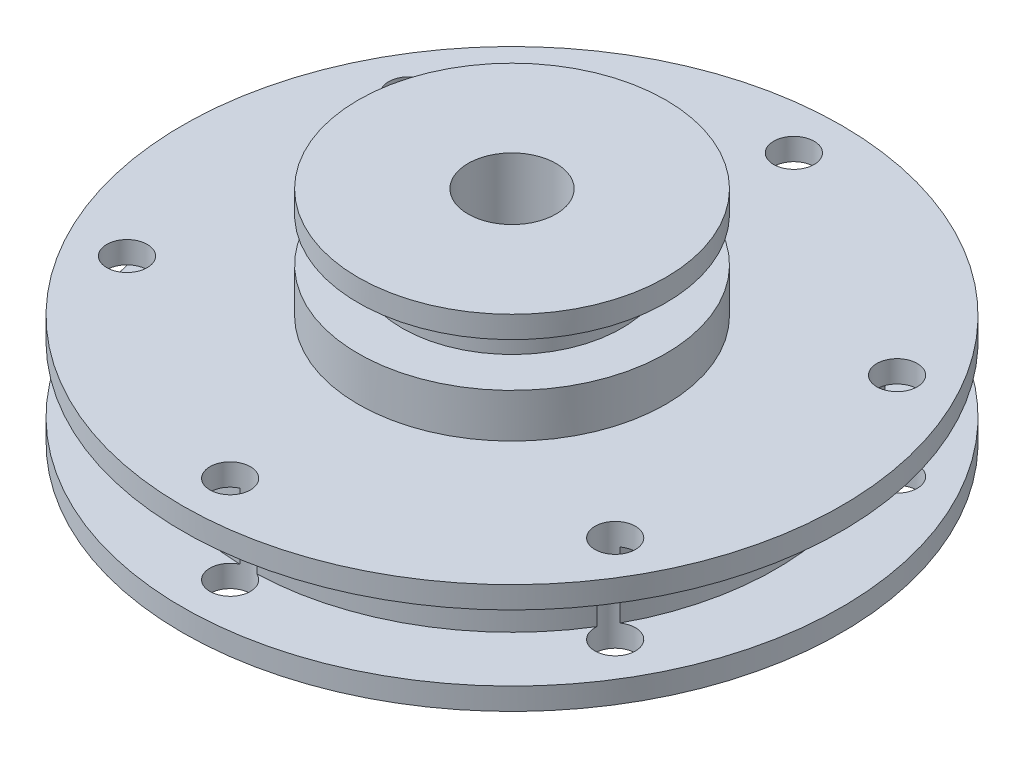
SolidWorks part; units mm, degrees
ref_plane "Front Plane" through (0, 0, 0) normal (0, 0, 1) x (1, 0, 0)
ref_plane "Top Plane" through (0, 0, 0) normal (0, 1, 0) x (1, 0, 0)
ref_plane "Right Plane" through (0, 0, 0) normal (1, 0, 0) x (0, 0, -1)
other "Configuration Table"
sketch "Sketch1" plane through (0, 0, 0) normal (0, 1, 0) x (1, 0, 0)
  circle A0 centre (0, 0) radius 15
  dimension "D1" = 30
extrude "Boss-Extrude1" add sketch "Sketch1" along normal blind 5
sketch "Sketch2" plane through (0, 0, 0) normal (0, 0, 1) x (1, 0, 0)
  line L0 (15, 0) -> (15, 5) construction
  line L1 (15, 4) -> (12, 4)
  line L2 (15, 4) -> (15, 1)
  line L3 (15, 1) -> (12, 1)
  line L4 (12, 4) -> (12, 1)
  line L5 (15, 5) -> (-15, 5) construction
  line L6 (0, 0) -> (0, 8.3794) construction
  line L7 (-15, 0) -> (15, 0) construction
  dimension "D1" = 3
  dimension "D2" = 3
  dimension "D3" = 1
revolve "Cut-Revolve1" cut sketch "Sketch2" angle 360 about L6
sketch "Sketch3" plane through (0, 5, 0) normal (0, 1, 0) x (1, 0, 0)
  circle A0 centre (0, 0) radius 7
  dimension "D1" = 14
extrude "Boss-Extrude2" add sketch "Sketch3" along normal blind 5
sketch "Sketch4" plane through (0, 0, 0) normal (0, 0, 1) x (1, 0, 0)
  line L0 (7, 5) -> (7, 10) construction
  line L1 (7, 9) -> (5, 9)
  line L2 (7, 9) -> (7, 7)
  line L3 (7, 7) -> (5, 7)
  line L4 (5, 9) -> (5, 7)
  line L5 (7, 10) -> (-7, 10) construction
  line L6 (0, 0) -> (0, 9.3794) construction
  dimension "D1" = 1
  dimension "D2" = 2
  dimension "D3" = 2
revolve "Cut-Revolve2" cut sketch "Sketch4" angle 360 about L6
sketch "Sketch5" plane through (0, 10, 0) normal (0, 1, 0) x (1, 0, 0)
  circle A0 centre (0, 0) radius 2
  dimension "D1" = 4
extrude "Cut-Extrude1" cut sketch "Sketch5" against normal through all
sketch "Sketch6" plane through (0, 5, 0) normal (0, 1, 0) x (1, 0, 0)
  circle A0 centre (0, 12.8299) radius 0.9206
  circle A1 centre (11.111, 6.4149) radius 0.9206
  circle A2 centre (11.111, -6.4149) radius 0.9206
  circle A3 centre (0, -12.8299) radius 0.9206
  circle A4 centre (-11.111, -6.4149) radius 0.9206
  circle A5 centre (-11.111, 6.4149) radius 0.9206
  point P14 (0, 0)
  dimension "D1" = 6
extrude "Cut-Extrude2" cut sketch "Sketch6" against normal through all both and the other way through all
